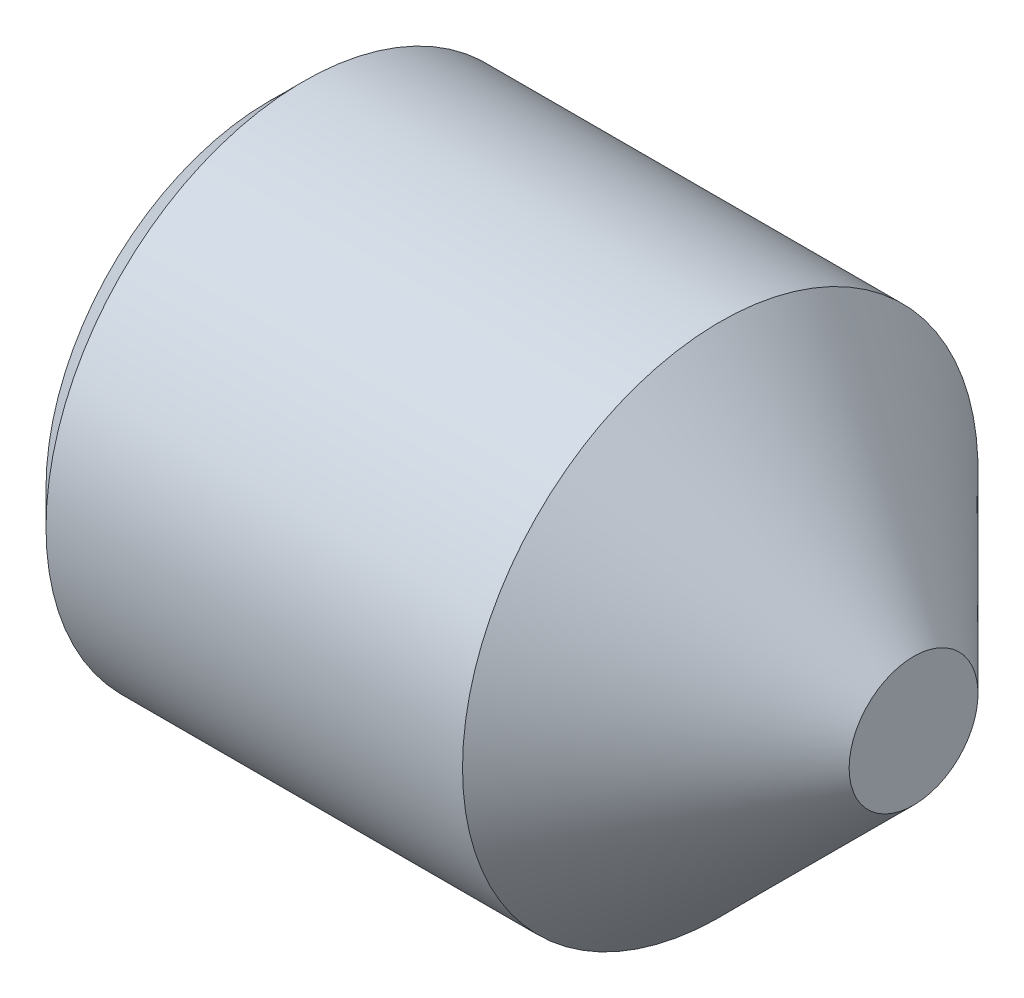
SolidWorks part; units mm, degrees
revolve "基体-旋转" add sketch "草图1" angle 360 about L0
sketch "草图1" plane through (0, 0, 0) normal (0, 0, 1) x (1, 0, 0)
  line L0 (-1.4105, 0) -> (5.3344, 0) construction
  line L1 (0, 0) -> (10, 0)
  line L2 (10, 0) -> (10, 1)
  line L3 (10, 1) -> (7, 4)
  line L4 (7, 4) -> (0.536, 4)
  line L5 (0.536, 4) -> (0, 3.464)
  line L6 (0, 3.464) -> (0, 0)
cosmetic thread "装饰螺纹线1" parameters "D1"=7, "df"=6.928
ref_plane "前视" through (0, 0, 0) normal (0, 0, 1) x (1, 0, 0)
ref_plane "上视" through (0, 0, 0) normal (0, 1, 0) x (1, 0, 0)
ref_plane "右视" through (0, 0, 0) normal (1, 0, 0) x (0, 0, -1)
sketch "尺寸草图" plane through (0, 0, 0) normal (0, 0, 1) x (1, 0, 0)
  line L0 (0, 0) -> (10, 0)
  point P3 (8, 0)
  point P4 (5.42, 0)
  point P5 (6.928, 0)
  point P6 (8, 0)
  point P7 (3, 0)
  point P8 (8.75, 0)
sketch "草图2" plane through (0, 0, 0) normal (-1, 0, 0) x (0, 0, 1)
  line L1 (2.29, 0) -> (1.145, 1.9832)
  line L2 (1.145, 1.9832) -> (-1.145, 1.9832)
  line L3 (-1.145, 1.9832) -> (-2.29, 0)
  line L4 (-2.29, 0) -> (-1.145, -1.9832)
  line L5 (-1.145, -1.9832) -> (1.145, -1.9832)
  line L6 (1.145, -1.9832) -> (2.29, 0)
  circle A0 centre (0, 0) radius 1.9832 construction
extrude "切除-拉伸1" cut sketch "草图2" against normal blind 3
sketch "草图3" plane through (0, 0, 0) normal (0, 0, 1) x (1, 0, 0)
  line L0 (3, 1.9832) -> (4.145, 0)
  line L1 (-1.4105, 0) -> (5.3344, 0) construction
  line L2 (4.145, 0) -> (3, 0)
  line L3 (3, 0) -> (3, 1.9832)
  line L4 (-0.1213, 0) -> (1.4124, 0) construction
  dimension "D1" = 60
revolve "切除-旋转1" cut sketch "草图3" angle 360 about L4
sketch "草图4" plane through (0, 0, 0) normal (0, 0, 1) x (1, 0, 0)
  line L0 (0.536, 4) -> (1.786, 4)
  line L1 (1.786, 4) -> (1.1542, 2.9175)
  line L2 (1.1542, 2.9175) -> (0.536, 4)
  line L3 (7, 4) -> (0.536, 4) construction
  line L5 (0.536, 4) -> (0.536, -4) construction
  line L6 (-0.1526, 0) -> (1.162, 0) construction
  line L7 (-1.4105, 0) -> (5.3344, 0) construction
revolve "切除-旋转2" [suppressed] cut sketch "草图4" angle 360 about L6
pattern_linear "阵列(线性)1" [suppressed] count 6
equation "\"l@草图1\" = \"l@尺寸草图\""
equation "\"d@草图1\" = \"d@尺寸草图\""
equation "\"df@草图1\" = \"df@尺寸草图\""
equation "\"dt@草图1\" = \"dt@尺寸草图\""
equation "\"df@装饰螺纹线1\" = \"df@尺寸草图\""
equation "\"e@草图2\" = \"e@尺寸草图\""
equation "\"t@切除-拉伸1\" = \"t@尺寸草图\""
equation "\"P@草图4\" = \"P@尺寸草图\""
equation "\"D1@草图4\" = \"P@尺寸草图\"*0.866"
equation "\"P@阵列(线性)1\" = \"P@尺寸草图\""
equation "\"D1@阵列(线性)1\" = (\"l@尺寸草图\"-\"d@尺寸草图\"/2+\"dt@尺寸草图\"/2)/\"P@尺寸草图\""
equation "\"D1@装饰螺纹线1\"=\"l@尺寸草图\"-\"d@尺寸草图\"/2+\"dt@尺寸草图\"/2"
